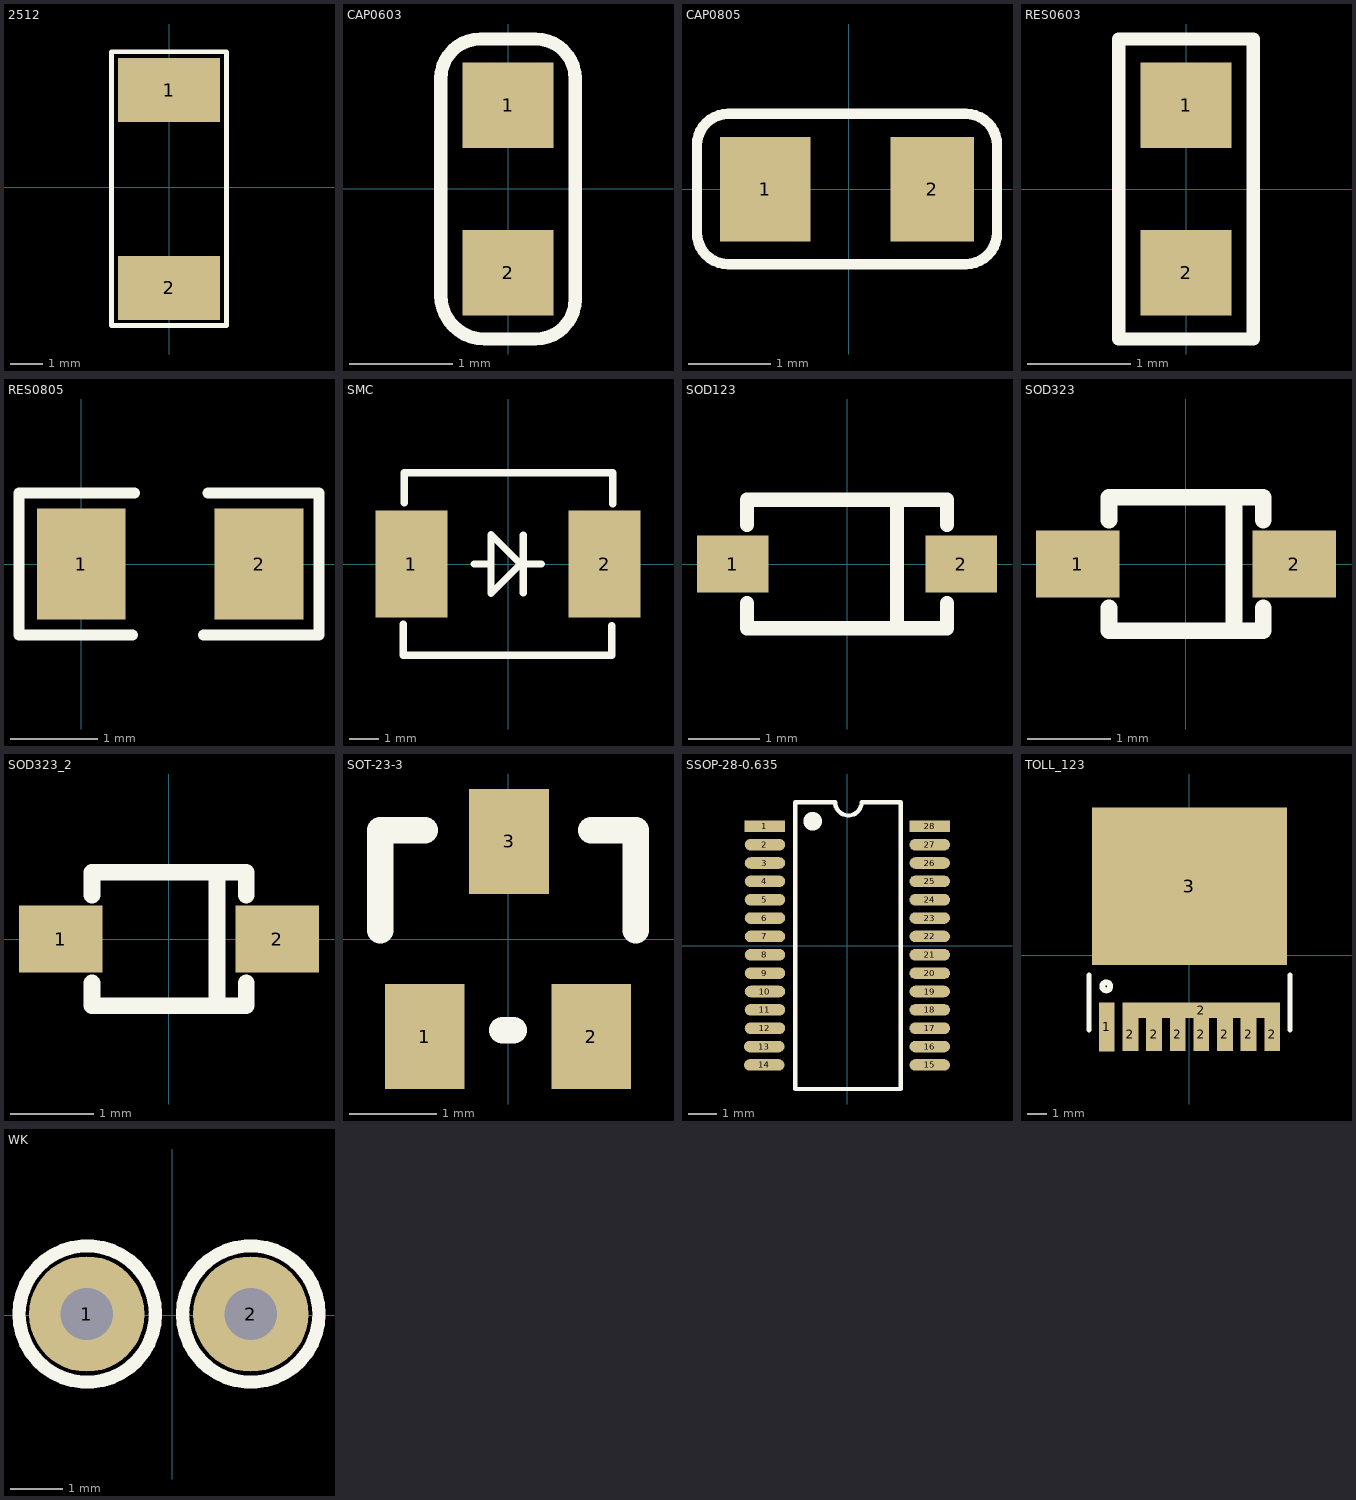
[diagram p0: the footprints below, top view; thin cyan lines are the x and y axes]
# Altium footprint library MISC84297-2.PcbLib: 13 footprints
Each footprint in its own frame and in the unit in brackets; x right, y up, seen from the top. Pads: shape width x height; smd on the part's side, far side on the other; paste and mask are expansions set on the pad; w line width, h text height; cw(c..) or ccw(c..) is an arc to the next point about the centre after c.

## 2512 [mm]
height 1.2
pads (2):
  rect 3.2x2 smd: 1(0,3.05) 2(0,-3.15)
Top Overlay:
  lines w0.15: -1.802,-4.325 -1.802,4.25 1.801,4.25 1.801,-4.325 -1.802,-4.325

## CAP0603 [mm] "CAP0402"
height 3.35
pads (2):
  rect 0.88x0.83 smd mask+0: 1(0,0.81) 2(0,-0.81)
Top Overlay:
  lines w0.127: -0.65,-1.027 ccw(c-0.227,-1.027) -0.227,-1.45 0.267,-1.45 ccw(c0.267,-1.067) 0.65,-1.067 0.65,1.067 ccw(c0.267,1.067) 0.267,1.45 -0.267,1.45 ccw(c-0.267,1.067) -0.65,1.067 -0.65,-1.027
3D body "0603_C.step": height 0.88, standoff 0, extent -0.412,-0.791 0.398,0.809

## CAP0805 [mil]
height 100
pads (2):
  rect 43.31x50 smd: 1(-40,0)
  rect 40x50 smd: 2(40,0)
Top Overlay:
  lines w5: 56,-35.96 -57.66,-35.96 cw(c-57.66,-21) -72.62,-21 -72.62,21 cw(c-57.66,21) -57.66,35.96 56,35.96 ; 56,-35.92 ccw(c56,-20.96) 70.96,-20.96 70.96,21.04 ccw(c56,21.04) 56,36
3D body "0805 SMD Capacitor.STEP": height 34.72, standoff 3.94, extent -39.36,-24.6 39.38,24.61

## RES0603 [mm] "CAP0402"
height 3.35
pads (2):
  rect 0.88x0.83 smd mask+0: 1(0,0.81) 2(0,-0.81)
Top Overlay:
  lines w0.127: 0.64,-1.45 -0.65,-1.45 -0.65,-0.4 -0.65,1.45 0.65,1.45 0.65,-0.44 ; 0.65,-1.45 0.65,-0.4
3D body "0603res.stp": height 0.3, standoff 0, extent -0.4,-0.83 0.4,0.77

## RES0805 [mil]
height 100
pads (2):
  rect 40x50 smd: 1(0,0) 2(80,0)
Top Overlay:
  lines w5: 23,-32 -28,-32 -28,32 24,32 ; 55,-32 107,-32 107,32 57,32
3D body "RES0805.STEP": height 3.94, standoff -12.2, extent 0.63,-25 79.37,24.21

## SMC [mm]
height 1.35
pads (2):
  rect 2.44x3.62 smd: 1(-3.275,0) 2(3.275,0)
Top Overlay:
  lines w0.25: -0.575,-1 0.425,0 -0.575,1 -0.575,-1
  lines w0.254: -3.55,-3.1 3.525,-3.1 3.525,-2.1 ; -3.55,-3.075 -3.55,-2.05 ; -3.525,2.075 -3.525,3.1 3.55,3.1 3.55,2.05 ; -1.15,0 -0.6,0 ; 0.5,0 1.125,0 ; 0.525,-0.975 0.525,0.025 ; 0.525,0 0.525,0.975

## SOD123 [mm]
height 2.45
pads (2):
  rect 1x0.8 smd: 1(-1.6,0) 2(1.6,0)
Top Overlay:
  lines w0.2: -1.4,-0.55 -1.4,-0.9 1.4,-0.9 1.4,-0.55 ; -1.4,0.55 -1.4,0.9 1.4,0.9 1.4,0.55 ; 0.7,-0.8 0.7,-0.5 0.7,0.8

## SOD323 [mm]
height 2.45
pads (2):
  rect 1x0.8 smd: 1(-1.3,0) 2(1.3,0)
Top Overlay:
  lines w0.2: -0.924,-0.525 -0.924,-0.8 0.926,-0.8 0.926,-0.525 ; -0.924,0.525 -0.924,0.8 0.926,0.8 0.926,0.525 ; 0.576,-0.8 0.576,-0.5 0.576,0.8

## SOD323_2 [mm]
pads (2):
  rect 1x0.8 smd: 1(-1.3,0) 2(1.3,0)
Top Overlay:
  lines w0.2: -0.924,-0.525 -0.924,-0.8 0.926,-0.8 0.926,-0.525 ; -0.924,0.525 -0.924,0.8 0.926,0.8 0.926,0.525 ; 0.576,-0.8 0.576,-0.5 0.576,0.8

## SOT-23-3 [mil]
height 55.12
pads (3):
  rect 36x47.24 smd: 1(-37.5,-43.94) 2(37.5,-43.94) 3(0.5,43.94)
Top Overlay:
  lines w12: -57.5,3.94 -57.5,48.94 -37.5,48.94 ; -2.5,-41.06 2.5,-41.06 ; 37.5,48.94 57.5,48.94 57.5,3.94

## SSOP-28-0.635 [mm]
height 1.4
pads (28):
  rect 1.4x0.4 smd: 1(-2.838,4.127) 28(2.862,4.127)
  oval 1.4x0.4 smd: 2(-2.838,3.492) 3(-2.838,2.857) 4(-2.838,2.222) 5(-2.838,1.587) 6(-2.838,0.953) 7(-2.838,0.318) 8(-2.838,-0.318) 9(-2.838,-0.953) 10(-2.838,-1.587) 11(-2.838,-2.222) 12(-2.838,-2.857) 13(-2.862,-3.492) 14(-2.862,-4.127) 15(2.862,-4.127) 16(2.862,-3.492) 17(2.862,-2.857) 18(2.862,-2.222) 19(2.862,-1.587) 20(2.862,-0.953) 21(2.862,-0.318) 22(2.862,0.318) 23(2.862,0.953) 24(2.862,1.587) 25(2.862,2.222) 26(2.862,2.857) 27(2.862,3.492)
Top Overlay:
  circle w0.5: c-1.188,4.303 r0.071
  lines w0.15: -1.787,4.96 -1.787,-4.96 1.863,-4.96 1.863,4.96 0.506,4.96 cw(c0.048,4.96) -0.41,4.96 -1.78,4.96

## TOLL_123 [mm] "SMD MOS"
height 3.35
pads (10):
  rect 0.8x2.5 smd: 1(-4.2,-3.638)
  rect 0.8x1.7 smd: 2(-3,-4) 2(-1.8,-4) 2(-0.6,-4) 2(0.6,-4) 2(1.8,-4) 2(3,-4) 2(4.2,-4)
  rect 8x0.8 smd: 2(0.6,-2.788)
  rect 9.9x8 smd: 3(0,3.5)
Top Overlay:
  circle w0.3: c-4.225,-1.575 r0.2
  lines w0.254: -5.1,-3.8 -5.1,-1 ; 5.1,-3.8 5.1,-1
Top Paste:
  region: -3.4,-3.03 -3.4,-2.39 4.6,-2.39 4.6,-3.08
  region: -4.95,7.5 4.95,7.5 4.95,-0.5 -4.95,-0.5
  region: -4.6,-4.85 -4.6,-3.15 -3.8,-3.15 -3.8,-4.85
  region: 3.8,-4.85 3.8,-3.25 4.6,-3.25 4.6,-4.85
  region: 2.6,-4.85 2.6,-3.25 3.4,-3.25 3.4,-4.85
  region: 1.4,-4.85 1.4,-3.25 2.2,-3.25 2.2,-4.85
  region: 0.2,-4.85 0.2,-3.25 1,-3.25 1,-4.85
  region: -1,-4.85 -1,-3.25 -0.2,-3.25 -0.2,-4.85
  region: -2.2,-4.85 -2.2,-3.25 -1.4,-3.25 -1.4,-4.85
  region: -3.4,-4.85 -3.4,-3.25 -2.6,-3.25 -2.6,-4.85

## WK [mm]
height 2.45
pads (2):
  round 2.2 hole 1: 1(-1.625,0.025) 2(1.5,0.025)
Top Overlay:
  circle w0.254: c-1.618,0.025 r1.3
  circle w0.254: c1.5,0.025 r1.3